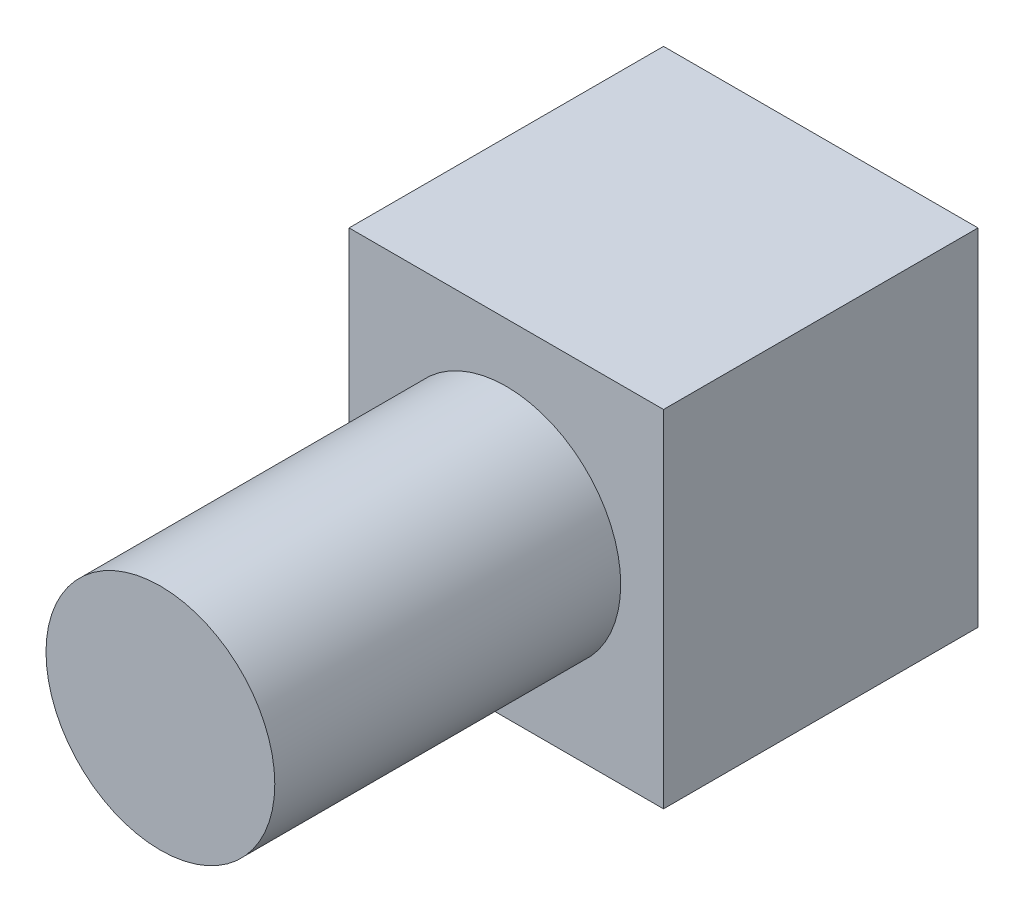
SolidWorks part; units mm, degrees
ref_plane "Front Plane" through (0, 0, 0) normal (0, 0, 1) x (1, 0, 0)
ref_plane "Top Plane" through (0, 0, 0) normal (0, 1, 0) x (1, 0, 0)
ref_plane "Right Plane" through (0, 0, 0) normal (1, 0, 0) x (0, 0, -1)
sketch "Sketch1" plane through (0, 0, 0) normal (0, 1, 0) x (1, 0, 0)
  line L1 (-25, 25) -> (25, 25)
  line L2 (-25, 25) -> (-25, -25)
  line L3 (-25, -25) -> (25, -25)
  line L4 (25, 25) -> (25, -25)
  line L5 (-25, 25) -> (25, -25) construction
  line L6 (-25, -25) -> (25, 25) construction
  point P0 (0, 0)
  dimension "D1" = 50
  dimension "D2" = 50
extrude "Boss-Extrude1" add sketch "Sketch1" along normal blind 55
sketch "Sketch2" plane through (0, 0, 25) normal (0, 0, 1) x (1, 0, 0)
  line L0 (-25, 55) -> (-25, 0) construction
  circle A0 centre (0, 27.5) radius 18.189
  point P4 (-25, 27.5)
extrude "Boss-Extrude2" add sketch "Sketch2" along normal blind 55
